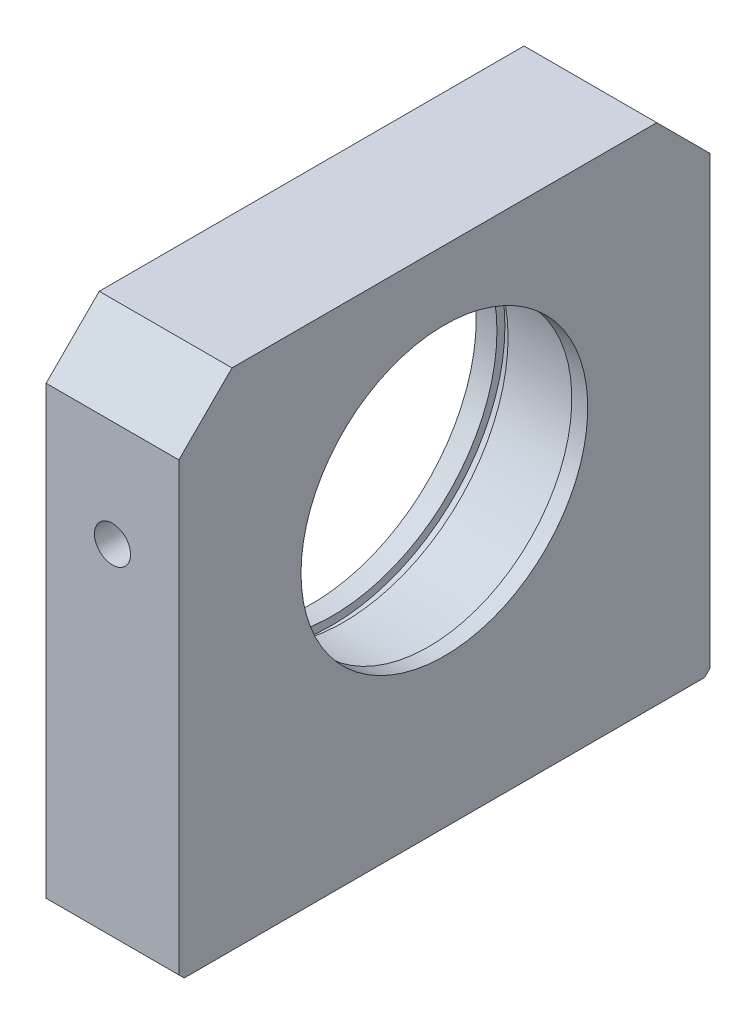
from build123d import *

# Parameters (mm, degrees)
SKETCH_1_W             = 100
SKETCH_1_H             = 95
EXTRUDE_1_DEPTH        = 25
SKETCH_2_R             = 31
CUT_EXTRUDE_1_DEPTH    = 22
SKETCH_3_R             = 27
CUT_EXTRUDE_2_DEPTH    = 73.389571072
CUT_EXTRUDE_START      = 16
SKETCH_4_R             = 32.5
CUT_EXTRUDE_3_DEPTH    = 2.1
HOLE_WIZARD_M8_1_D     = 6.8
HOLE_WIZARD_M8_1_DEPTH = 15.75
HOLE_WIZARD_M8_1_TIP   = 2.042926105
HOLE_WIZARD_M8_2_D     = 6.8
HOLE_WIZARD_M8_2_DEPTH = 15.75
HOLE_WIZARD_M8_2_TIP   = 2.042926105
CHAMFER_1_SIZE         = 10
CHAMFER_2_SIZE         = 1
HOLE_WIZARD_M8_3_D     = 6.8
HOLE_WIZARD_M8_3_DEPTH = 19.75
HOLE_WIZARD_M8_3_TIP   = 2.042926105


with BuildPart() as part:
    # 草图1 → 凸台-拉伸1 (new body)
    with BuildSketch(Plane(origin=(0, 0, 0), x_dir=(0, 0, -1), z_dir=(1, 0, 0))):
        Rectangle(SKETCH_1_W, SKETCH_1_H)
    extrude(amount=EXTRUDE_1_DEPTH)

    # 草图2 → 切除-拉伸1 (cut)
    with BuildSketch(Plane.ZY):
        with Locations((0, 7.5)):
            Circle(SKETCH_2_R)
    extrude(amount=-CUT_EXTRUDE_1_DEPTH, mode=Mode.SUBTRACT)

    # 草图3 → 切除-拉伸2 (cut, through all)
    with BuildSketch(Plane.ZY.offset(-22)):
        with Locations((0, 7.5)):
            Circle(SKETCH_3_R)
    extrude(amount=-CUT_EXTRUDE_2_DEPTH, mode=Mode.SUBTRACT)

    # 草图4 → 切除-拉伸3 (cut)
    with BuildSketch(Plane.ZY.offset(-22).offset(CUT_EXTRUDE_START)):
        with Locations((0, 7.5)):
            Circle(SKETCH_4_R)
    extrude(amount=CUT_EXTRUDE_3_DEPTH, mode=Mode.SUBTRACT)

    # M8 螺纹孔1
    with Locations(Plane.XY.offset(50)):
        with Locations((12.5, 17.5)):
            Hole(HOLE_WIZARD_M8_1_D / 2, depth=HOLE_WIZARD_M8_1_DEPTH)
            with Locations((0, 0, -(HOLE_WIZARD_M8_1_DEPTH + HOLE_WIZARD_M8_1_TIP / 2))):  # 118° drill point
                Cone(0, HOLE_WIZARD_M8_1_D / 2, HOLE_WIZARD_M8_1_TIP, mode=Mode.SUBTRACT)

    # M8 螺纹孔2
    with Locations(Plane(origin=(0, 0, -50), x_dir=(-1, 0, 0), z_dir=(0, 0, -1))):
        with Locations((-12.5, 17.5)):
            Hole(HOLE_WIZARD_M8_2_D / 2, depth=HOLE_WIZARD_M8_2_DEPTH)
            with Locations((0, 0, -(HOLE_WIZARD_M8_2_DEPTH + HOLE_WIZARD_M8_2_TIP / 2))):  # 118° drill point
                Cone(0, HOLE_WIZARD_M8_2_D / 2, HOLE_WIZARD_M8_2_TIP, mode=Mode.SUBTRACT)

    # 倒角1
    chamfer_1_edges = [part.edges().sort_by_distance(p)[0] for p in [
        (12.5, 47.5, 50),
        (12.5, 47.5, -50),
    ]]
    chamfer(chamfer_1_edges, length=CHAMFER_1_SIZE)

    # 倒角2
    chamfer_2_edges = [part.edges().sort_by_distance(p)[0] for p in [
        (12.5, -47.5, -50),
        (12.5, -47.5, 50),
    ]]
    chamfer(chamfer_2_edges, length=CHAMFER_2_SIZE)

    # M8 螺纹孔3
    with Locations(Plane(origin=(0, -47.5, 0), x_dir=(-1, 0, 0), z_dir=(0, -1, 0))):
        with Locations((-12.5, -40), (-12.5, 0), (-12.5, 40)):
            Hole(HOLE_WIZARD_M8_3_D / 2, depth=HOLE_WIZARD_M8_3_DEPTH)
            with Locations((0, 0, -(HOLE_WIZARD_M8_3_DEPTH + HOLE_WIZARD_M8_3_TIP / 2))):  # 118° drill point
                Cone(0, HOLE_WIZARD_M8_3_D / 2, HOLE_WIZARD_M8_3_TIP, mode=Mode.SUBTRACT)


solid = part.part
